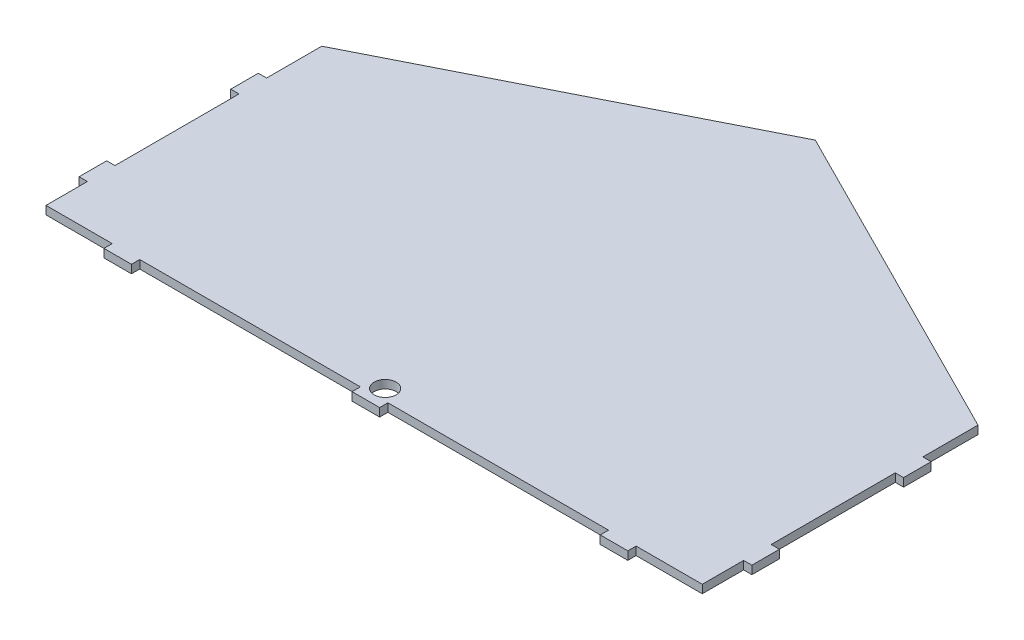
from build123d import *

# Parameters (mm, degrees)
BOSS_EXTRUDE1_DEPTH = 3
SKETCH3_W           = 3
SKETCH3_H           = 10
SKETCH3_W_2         = 10
SKETCH3_H_2         = 3
BOSS_EXTRUDE2_DEPTH = 3
SKETCH4_R           = 4
CUT_EXTRUDE1_DEPTH  = 165.295465549


with BuildPart() as part:
    # Sketch1 → Boss-Extrude1 (new body)
    with BuildSketch(Plane(origin=(0, 0, 0), x_dir=(1, 0, 0), z_dir=(0, 1, 0))):
        Polygon((-119, 50), (0, 110), (119, 50), (119, -50), (-119, -50), align=None)
    extrude(amount=BOSS_EXTRUDE1_DEPTH)

    # Sketch3 → Boss-Extrude2 (add)
    with BuildSketch(Plane(origin=(0, 3, 0), x_dir=(1, 0, 0), z_dir=(0, 1, 0))):
        with Locations((120.5, 25)):
            Rectangle(SKETCH3_W, SKETCH3_H)
        with Locations((120.5, -30)):
            Rectangle(SKETCH3_W, SKETCH3_H)
        with Locations((-120.5, -30)):
            Rectangle(SKETCH3_W, SKETCH3_H)
        with Locations((-120.5, 25)):
            Rectangle(SKETCH3_W, SKETCH3_H)
        with Locations((-90, -51.5)):
            Rectangle(SKETCH3_W_2, SKETCH3_H_2)
        with Locations((90, -51.5)):
            Rectangle(SKETCH3_W_2, SKETCH3_H_2)
        with Locations((0, -51.5)):
            Rectangle(SKETCH3_W_2, SKETCH3_H_2)
    extrude(amount=-BOSS_EXTRUDE2_DEPTH)

    # Sketch4 → Cut-Extrude1 (cut, through all)
    with BuildSketch(Plane(origin=(0, 3, 0), x_dir=(1, 0, 0), z_dir=(0, 1, 0))):
        with Locations(Location((0, -46, 0), (0, 0, 270))):
            Circle(SKETCH4_R)
    extrude(amount=-CUT_EXTRUDE1_DEPTH, mode=Mode.SUBTRACT)


solid = part.part
